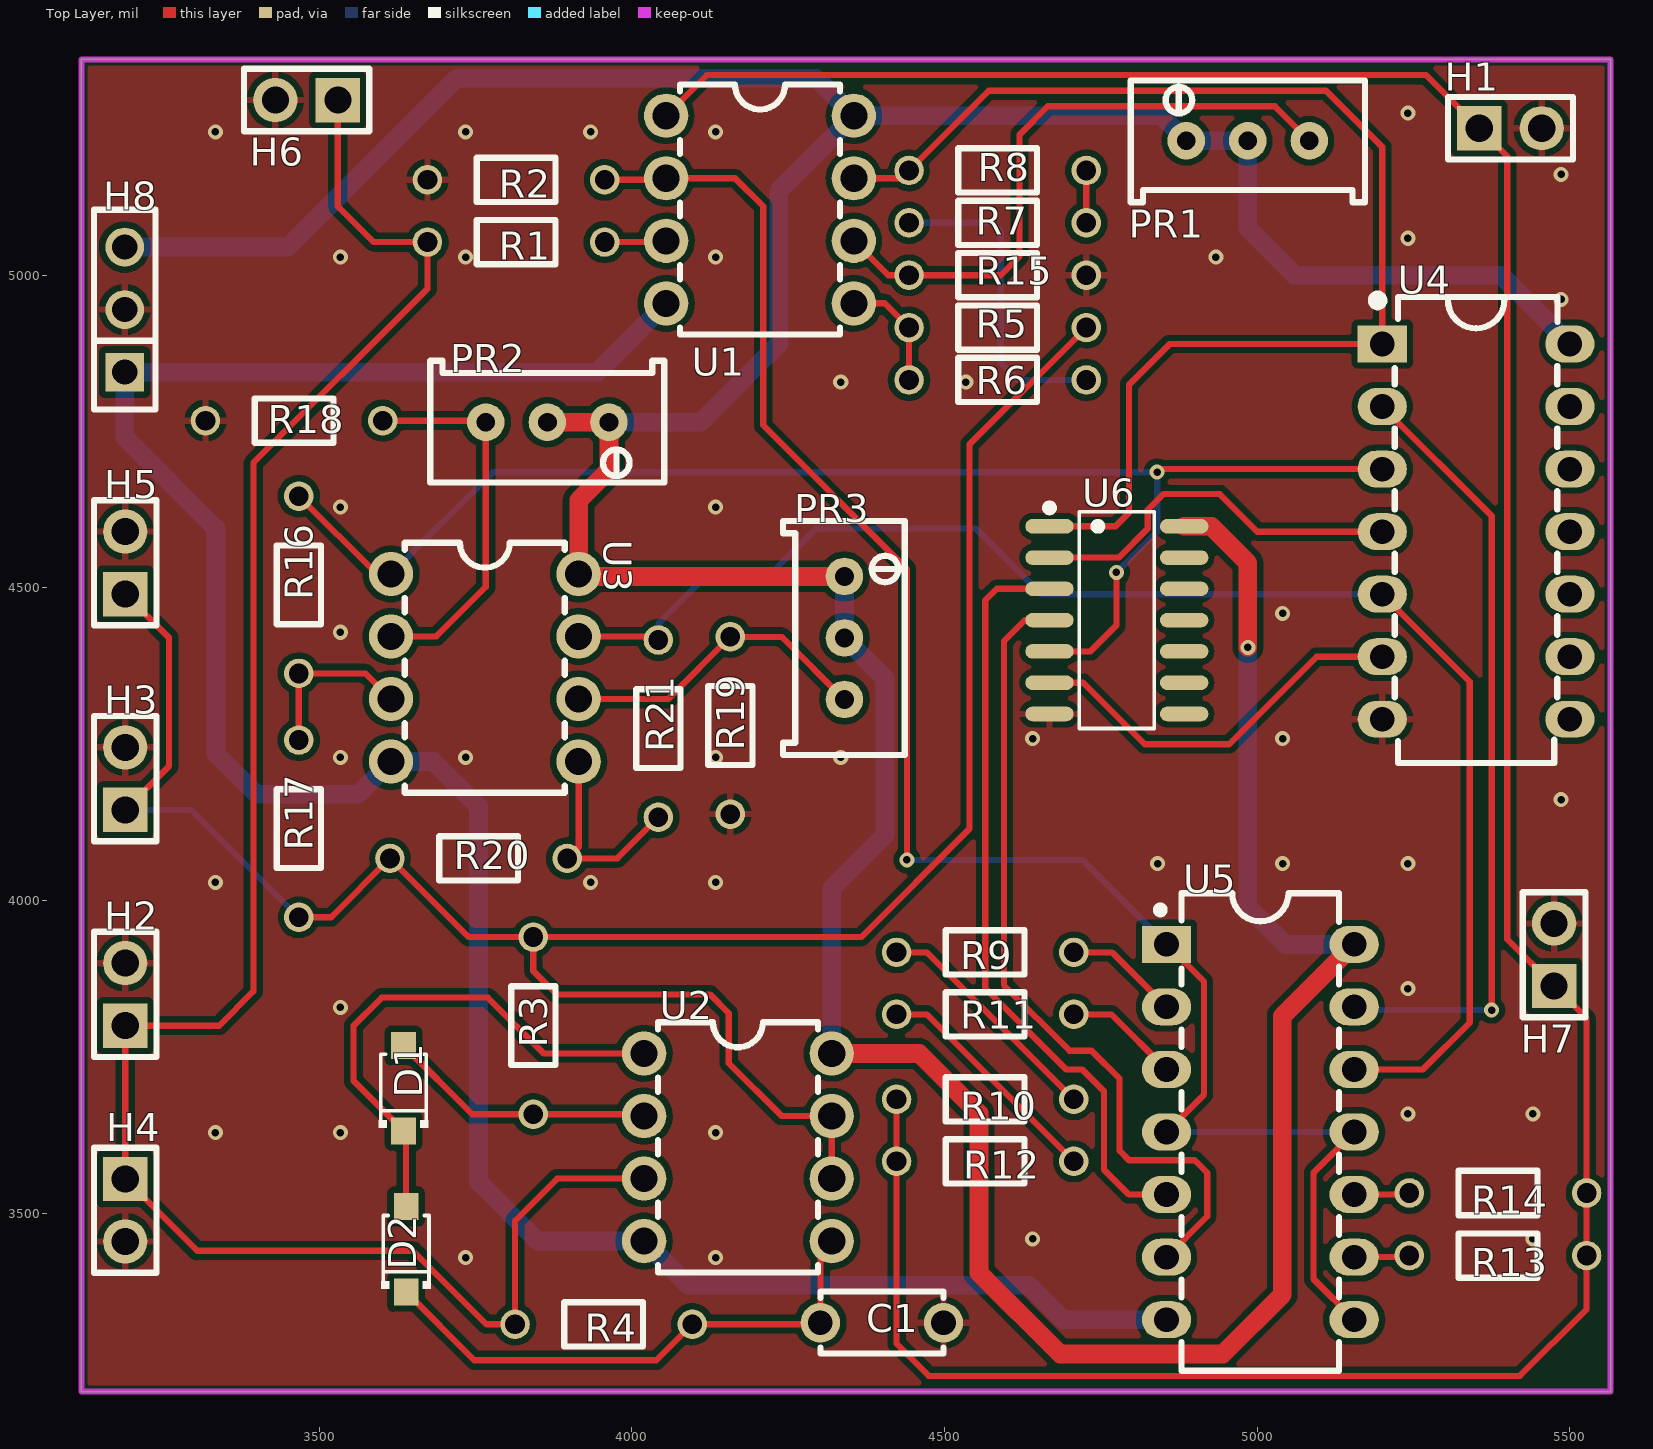
[diagram p0: Top Layer view]
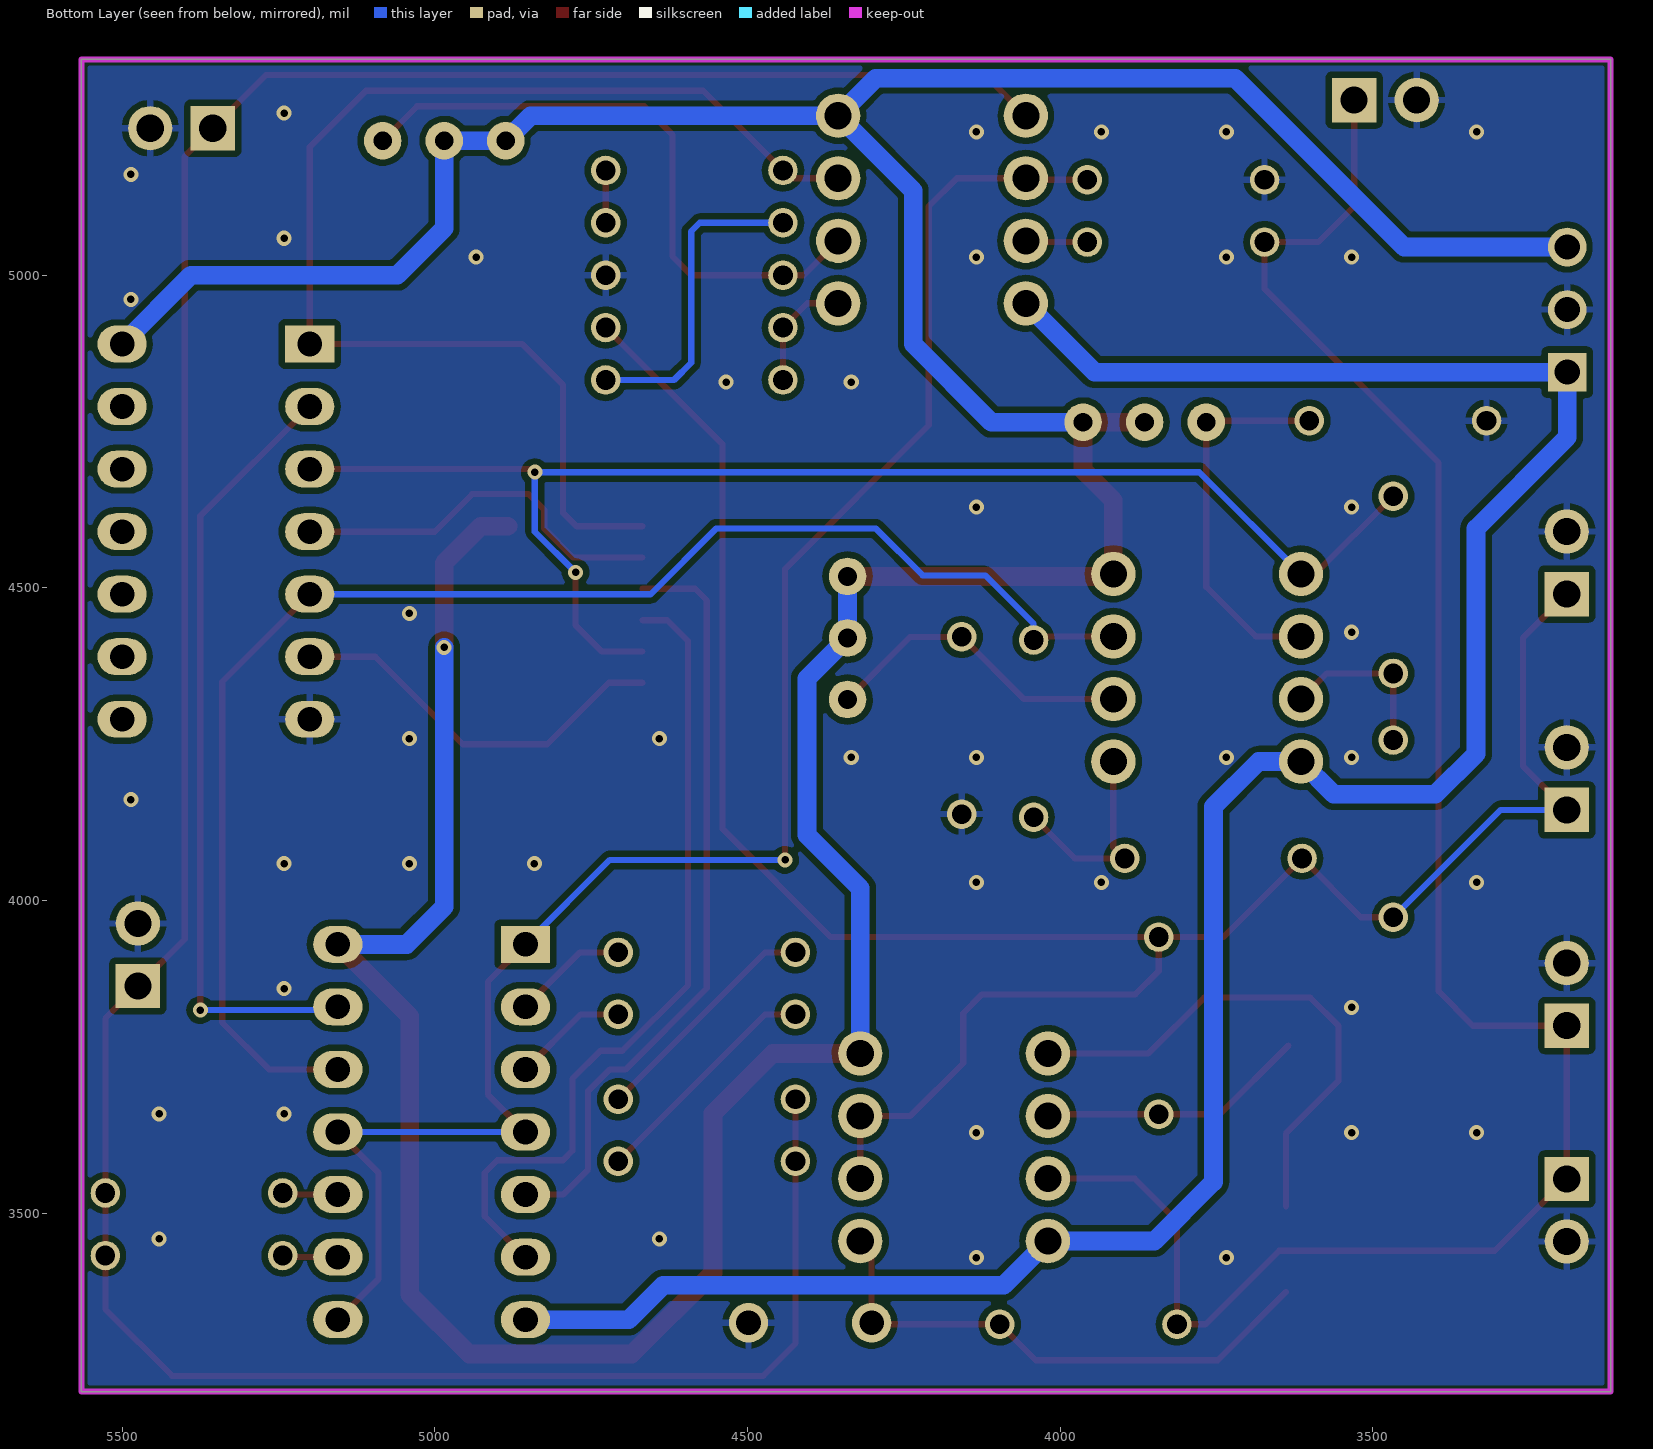
[diagram p1: Bottom Layer view, seen from below]
# Altium PCB MISC51795.pcbdoc
Units mil, origin at the board's own origin, x right, y up, seen from the top; angles counter-clockwise.
Board outline 2445 x 2130 mil, 2 copper layers (Top Layer, Bottom Layer), stack 62.206 mil thick; 41 components, 39 nets, 140 pads, 47 vias.

## Layer stack, top to bottom
Top Solder Mask Layer: solder mask 0.394, Dk 3.3
Top Layer: signal copper 1.379
Dielectric1: surface 59.449, FR4, Dk 4.5
Bottom Layer: signal copper 1.378
Bottom Solder Mask Layer: solder mask 0.394, Dk 3.3

## Board outline
3120,5345 3120,3215 5565,3215 5565,5345

## Design rules (kind name [scope] priority, off if disabled: settings)
BoardOutlineClearance copperThickness2oz_1 [All] p2 off: genericclearance=7.99 ignorepadtopadclearanceinfootprint=FALSE except(0: Arc-SplitContinuation Track-SplitContinuation SMDPad-SplitContinuation THPad-SplitContinuation Via-SplitContinuation Fill-SplitContinuation Region-SplitContinuation Poly-SplitContinuation Text-SplitContinuation Hole-SplitContinuation; 5.98: Arc-CutoutEdge SMDPad-CutoutEdge THPad-CutoutEdge Via-CutoutEdge Fill-CutoutEdge Region-CutoutEdge Text-CutoutEdge; 6.93: Hole-OutlineEdge Hole-CutoutEdge; 10: Poly-OutlineEdge Poly-CutoutEdge; 11.81: Arc-OutlineEdge Track-OutlineEdge SMDPad-OutlineEdge THPad-OutlineEdge Via-OutlineEdge Fill-OutlineEdge Region-OutlineEdge Text-OutlineEdge Track-CutoutEdge)
BoardOutlineClearance copperThickness1oz_1 [All] p4: genericclearance=4.02 ignorepadtopadclearanceinfootprint=FALSE except(0: Arc-SplitContinuation Track-SplitContinuation SMDPad-SplitContinuation THPad-SplitContinuation Via-SplitContinuation Fill-SplitContinuation Region-SplitContinuation Poly-SplitContinuation Text-SplitContinuation Hole-SplitContinuation; 6: SMDPad-CutoutEdge THPad-CutoutEdge Via-CutoutEdge Fill-CutoutEdge Region-CutoutEdge Text-CutoutEdge; 6.93: Hole-OutlineEdge Hole-CutoutEdge; 10: Poly-OutlineEdge Poly-CutoutEdge; 11.8: Arc-OutlineEdge Track-OutlineEdge SMDPad-OutlineEdge THPad-OutlineEdge Via-OutlineEdge Fill-OutlineEdge Region-OutlineEdge Text-OutlineEdge; 11.81: Arc-CutoutEdge Track-CutoutEdge)
Clearance copperThickness2oz [All] p1 off: gap=7.99 ignorepadtopadclearanceinfootprint=FALSE except(5.98: SMDPad-Track SMDPad-SMDPad THPad-Track SMDPad-THPad THPad-THPad Track-Via SMDPad-Via THPad-Via Via-Via Fill-Track Region-Track Fill-SMDPad Region-SMDPad Fill-THPad Region-THPad Fill-Via Region-Via Fill-Fill Fill-Region Region-Region Arc-Track Arc-SMDPad Arc-THPad Arc-Via Fill-Arc Region-Arc Arc-Arc Text-Track SMDPad-Text Text-THPad Text-Via Fill-Text Region-Text Arc-Text Text-Text; 6.93: Hole-Track Hole-SMDPad Hole-THPad Hole-Via Fill-Hole Region-Hole Hole-Arc Hole-Text; 10: Poly-Track Poly-SMDPad Poly-THPad Poly-Via Poly-Fill Poly-Region Poly-Poly Poly-Arc Poly-Text Poly-Hole)
Clearance copperThickness1oz [All] p3: gap=4.02 ignorepadtopadclearanceinfootprint=FALSE except(5.98: SMDPad-Track SMDPad-SMDPad THPad-Track SMDPad-THPad THPad-THPad Track-Via SMDPad-Via THPad-Via Via-Via Fill-Track Region-Track Fill-SMDPad Region-SMDPad Fill-THPad Region-THPad Fill-Via Region-Via Fill-Fill Fill-Region Region-Region; 6: Arc-Track Arc-SMDPad Arc-THPad Arc-Via Fill-Arc Region-Arc Arc-Arc Text-Track SMDPad-Text Text-THPad Text-Via Fill-Text Region-Text Arc-Text Text-Text; 6.93: Hole-Track Hole-SMDPad Hole-THPad Hole-Via Fill-Hole Region-Hole Hole-Arc Hole-Text; 10: Poly-Track Poly-SMDPad Poly-THPad Poly-Via Poly-Fill Poly-Region Poly-Poly Poly-Arc Poly-Text Poly-Hole)
Creepage creepage [All] p1: checkdistance=0 ignoreinternallayers=TRUE applytopolygonpour=TRUE
DiffPairsRouting differentialPair [All] p1: maxlimit=6 minlimit=6 mostfreqgap=6 toplayer_minwidth=5 toplayer_prefwidth=10 toplayer_maxwidth=100 toplayer_mingap=6 toplayer_prefgap=6 toplayer_maxgap=6 bottomlayer_minwidth=5 bottomlayer_prefwidth=10 bottomlayer_maxwidth=100 bottomlayer_mingap=6 bottomlayer_prefgap=6 bottomlayer_maxgap=6 maxuncoupledlength=10
HoleToHoleClearance otherClearance [All] p1: gap=11.81 allowstackedmicrovias=TRUE
Length netLength [All] p1: minlimit=0 maxlimit=0
MatchedLengths netLengthTolerance [All] p1: tolerance=1000
PasteMaskExpansion pasteMaskExpansion [All] p1: expansion=0
PlaneConnect innerPlane [All] p1: planeconnectstyle=Relief reliefexpansion=20 reliefentries=4 reliefconductorwidth=10 reliefairgap=10
PolygonConnect copperRegion [(InNet('GND'))] p1: connectstyle=Relief reliefconductorwidth=10 reliefentries=4 polygonreliefangle="90 Angle" airgapwidth=10 via.connectstyle=Relief via.reliefconductorwidth=10 via.reliefentries=4 via.polygonreliefangle="90 Angle" via.airgapwidth=10
RoutingVias viaSize [All] p1: holewidth=12.01 width=24.02 viastyle="Through Hole" minholewidth=11.81 minwidth=19.68 maxholewidth=248.03 maxwidth=393.7
SolderMaskExpansion solderMaskExpansion [IsVia] p1: expansion=-1000 istentingtop=TRUE
SolderMaskExpansion solderMaskExpansion [All] p2: expansion=2 istentingtop=FALSE
Width copperThickness2oz_2 [All] p1 off: maxlimit=100 minlimit=8 preferedwidth=10
Width copperThickness1oz_2 [All] p2: maxlimit=100 minlimit=5 preferedwidth=10

## Components (designator, comment, footprint, x,y, rotation, side; value= is the part's Value field where it differs from the comment)
C1 "22uF" CAP-TH_L5.0-W2.5-P5.00-D1.0 4400,3325 r180 top
D1 "1N4148W" SOD-123F_L2.7-W1.6-LS3.8-RD 3635,3700 r90 top
D2 "1N4148W" SOD-123F_L2.7-W1.6-LS3.8-RD 3639.08,3442.49 r90 top
H1 "" HDR-TH_2P-P2.54-V-M-1 5405,5235 r0 top
H2 "" HDR-TH_2P-P2.54-V-M-1 3190,3850.04 r90 top
H3 "" HDR-TH_2P-P2.54-V-M-1 3190,4195.08 r90 top
H4 "" HDR-TH_2P-P2.54-V-M-1 3190,3505 r270 top
H5 "" HDR-TH_2P-P2.54-V-M-1 3190,4540.12 r90 top
H6 "" HDR-TH_2P-P2.54-V-M-1 3480,5280 r180 top
H7 "" HDR-TH_2P-P2.54-V-M-1 5474.79,3913.46 r90 top
H8 "" HDR-TH_3P-P2.54-V-F 3189.21,4945 r90 top
PR1 "51kΩ" R_3296 4985,5220 r0 top
PR2 "51kΩ" R_3296 3865,4760 r180 top
PR3 "51kΩ" R_3296 4345,4420 r270 top
R1 "10K" Res_1/8W 3815,5050.47 r0 top
R2 "10K" Res_1/8W 3815,5150 r0 top
R3 "1K" Res_1/8W 3845,3800 r90 top
R4 "10K" Res_1/8W 3955,3320 r0 top
R5 "1K" Res_1/8W 4585,4918.71 r180 top
R6 "100K" Res_1/8W 4585,4830 r0 top
R7 "82K" Res_1/8W 4585,5081.29 r0 top
R8 "5.1K" Res_1/8W 4585,5170 r180 top
R9 "45K" Res_1/8W 4565.05,3919.68 r180 top
R10 "5.1K" Res_1/8W 4565.05,3684.68 r180 top
R11 "39K" Res_1/8W 4565.05,3820.56 r180 top
R12 "1K" Res_1/8W 4565.05,3585.56 r180 top
R13 "20K" Res_1/8W 5385,3430 r0 top
R14 "9.5K" Res_1/8W 5385,3530 r0 top
R15 "2K" Res_1/8W 4585,5002.48 r180 top
R16 "75K" Res_1/8W 3470,4505 r90 top
R17 "1K" Res_1/8W 3470,4115 r90 top
R18 "2K" Res_1/8W 3460,4765 r0 top
R19 "2K" Res_1/8W 4160,4280 r90 top
R20 "1K" Res_1/8W 3755,4065 r0 top
R21 "75K" Res_1/8W 4045,4275 r90 top
U1 "LM358AP" PDIP-8_L10.2-W6.5-P2.54-LS7.6-BL 4205,5105 r270 top
U2 "LM358AN/NOPB" PDIP-8_L10.2-W6.5-P2.54-LS7.6-BL 4169.69,3605.56 r270 top
U3 "LM358AN/NOPB" PDIP-8_L10.2-W6.5-P2.54-LS7.6-BL 3765,4372.38 r270 top
U4 "CD40106BD" DIP-14_L19.1-W6.4-P2.54-LS7.6-BL 5350,4590 r270 top
U5 "SN74LV4066AN" PDIP-14_L19.3-W6.4-P2.54-LS7.9-BL-1 5005,3630 r270 top
U6 "HEF4081BT118" SO-14_L8.9-W3.9-P1.27-LS6.0-BL 4775.51,4448.46 r270 top

## Footprints (in the part's own frame and the unit in brackets; to place one, negate y for a bottom-side part, rotate by r counter-clockwise, add the part's x,y. Pads: shape width x height; smd on the part's side, far side on the other; paste and mask are expansions set on the pad)
CAP-TH_L5.0-W2.5-P5.00-D1.0 [mm]
  round 1.6 hole 1: 1(-2.5,0) 2(2.5,0)
  silkscreen extent -2.5,-1.27 2.5,1.25
DIP-14_L19.1-W6.4-P2.54-LS7.6-BL [mm]
  rect 1.5x2 hole 1: 1(-7.62,-3.81)
  oval 1.5x2 hole 1: 2(-5.08,-3.81) 3(-2.54,-3.81) 4(0,-3.81) 5(2.54,-3.81) 6(5.08,-3.81) 7(7.62,-3.81) 8(7.62,3.81) 9(5.08,3.81) 10(2.54,3.81) 11(0,3.81) 12(-2.54,3.81) 13(-5.08,3.81) 14(-7.62,3.81)
  silkscreen extent -9.59,-4.2 9.4,3.3
HDR-TH_2P-P2.54-V-M-1 [mm]
  rect 1.8x1.8 hole 1.1: 1(-1.27,0)
  round 1.8 hole 1.1: 2(1.27,0)
  silkscreen extent -2.54,-1.27 2.54,1.27
HDR-TH_3P-P2.54-V-F [mil]
  rect 62x62 hole 40.16: 1(-100,0)
  round 62 hole 40.16: 2(0,0) 3(100,0)
  silkscreen extent -160,-49 160,49
PDIP-8_L10.2-W6.5-P2.54-LS7.6-BL [mm]
  round 1.8 hole 1.1: 1(-3.81,-3.81) 2(-1.27,-3.81) 3(1.27,-3.81) 4(3.81,-3.81) 5(3.81,3.81) 6(1.27,3.81) 7(-1.27,3.81) 8(-3.81,3.81)
  silkscreen extent -5.08,-3.25 5.08,3.25
PDIP-14_L19.3-W6.4-P2.54-LS7.9-BL-1 [mm]
  rect 1.5x2 hole 1: 1(-7.62,-3.81)
  oval 1.5x2 hole 1: 2(-5.08,-3.81) 3(-2.54,-3.81) 4(0,-3.81) 5(2.54,-3.81) 6(5.08,-3.81) 7(7.62,-3.81)
  oval 1.5x2 hole 1 copper offset 0,0: 8(7.62,3.81) 9(5.08,3.81) 10(2.54,3.81) 11(0,3.81) 12(-2.54,3.81) 13(-5.08,3.81) 14(-7.62,3.81)
  silkscreen extent -9.7,-4.21 9.7,3.2
R_3296 [mil]
  round 60 hole 30 paste+0 mask+2: 1(-98.4,-5) 2(0,-5) 3(98.4,-5)
  silkscreen extent -187,-103 187,92
Res_1/8W [mil]
  round 47.2 hole 31.5 paste+0 mask+2: 1(-141.7,2.48) 2(141.7,2.48)
  silkscreen extent -63,-33 63,38
SO-14_L8.9-W3.9-P1.27-LS6.0-BL [mm]
  oval 0.595x1.968 smd: 1(-3.81,-2.734) 2(-2.54,-2.734) 3(-1.27,-2.734) 4(0,-2.734) 5(1.27,-2.734) 6(2.54,-2.734) 7(3.81,-2.734) 8(3.81,2.734) 9(2.54,2.734) 10(1.27,2.734) 11(0,2.734) 12(-1.27,2.734) 13(-2.54,2.734) 14(-3.81,2.734)
  silkscreen extent -4.71,-2.88 4.4,1.52
SOD-123F_L2.7-W1.6-LS3.8-RD [mm]
  rect 1.1x1 smd: 1(-1.735,0) 2(1.735,0)
  silkscreen extent -1.6,-1 1.38,1

## Via types
v1: diameter 24.02, hole 12, Top Layer to Bottom Layer, 47 vias

## Nets (pads, with @x,y where several pads share a name; then routed paths per layer and width w, separated by ;. In a path a pad name is that pad's centre, name@x,y a point inside that pad or via, vN(x,y) a via of type N, cw(c..) or ccw(c..) an arc to the next point about the centre after c; other vN are vias at no path point)
9V: H8.3 PR1.1 PR1.2 PR2.1 PR2.2 PR3.1 PR3.2 U1.8 U2.8 U3.8 U4.14 U5.14 U6.14 | length 7618.2
  Top Layer w30: PR2.2 PR2.1 3963.4,4688.4 3915,4640 U3.8 3918.98,4518.4 PR3.1 ; U2.8 4459.44,3755.56 4555,3660 4555,3405 4685,3275 4945,3275 5040,3370 5040,3815 U5.14 ; U6.14 4926.54,4598.46 4985,4540 v1(4985,4405)
  Bottom Layer w30: H8.3 3450,5045 3720,5315 4295,5315 U1.8 ; PR2.1 4110,4765 4235,4890 4235,5135 U1.8 ; U2.8 4319.69,4019.68 4405,4105 4405,4355 PR3.2 PR3.1 ; v1(4985,4405) 4985,3990 5045,3930 U5.14 ; U4.14 5390,5000 5060,5000 4985,5075 PR1.2 PR1.1 4846.6,5255 U1.8
$1N4: R1.2 U1.3 | length 99.2
  Top Layer w10: R1.2 4052.95,5052.95 U1.3
$1N7: H2.1 H4.1 H6.1 R1.1 R4.1 U2.3 | length 3242.6
  Top Layer w10: H6.1 3530,5110 3587.05,5052.95 R1.1 3673.3,4978.3 3395,4700 3395,3855 3340.04,3800.04 H2.1 H4.1 3305,3440 3650,3440 3767.52,3322.48 R4.1 3813.3,3488.3 3880.56,3555.56 U2.3
$1N12: D1.2 R3.1 U2.2 | length 431.4
  Top Layer w10: D1.2 3745.01,3658.3 R3.1 4016.94,3658.3 U2.2
$1N13: D1.1 D2.2 U2.1 | length 844.4
  Top Layer w10: D2.2 3639.08,3627.62 D1.1 3555,3711.7 3555,3800 3600,3845 3770,3845 3859.44,3755.56 U2.1
$1N14: C1.2 D2.1 R4.2 U2.5 | length 870.6
  Top Layer w10: D2.1 3748.26,3265 4039.22,3265 R4.2 4299.05,3322.48 C1.2 4301.57,3437.45 U2.5
$1N21: R5.2 R6.1 U1.5 | length 188.1
  Top Layer w10: U1.5 4404.54,4955 R5.2 R6.1
$1N22: R6.2 R7.1 | length 510.5
  Bottom Layer w10: R7.1 4576.24,5083.76 4590,5070 4590,4860 4617.52,4832.48 R6.2
$1N24: R7.2 R8.1 | length 83.8
  Top Layer w10: R7.2 R8.1
$1N26: PR1.3 R15.2 U1.6 | length 1000
  Top Layer w10: U1.6 4410,5000 R15.2 4590,5000 4620,5030 4620,5225 4665,5270 5028.4,5270 PR1.3
$1N44: R2.2 U1.2 U5.1 U5.4 U5.8 U5.11 | length 2887.7
  Top Layer w10: R2.2 4052.48,5152.48 U1.2 4165,5155 4210,5110 4210,4760 4440,4530 v1(4440,4065) ; U5.4 4915,3690 4915,3870.01 U5.1 ; U5.8 5090,3395 5090,3565 U5.11
  Bottom Layer w10: v1(4440,4065) 4720.01,4065 U5.1 ; U5.4 U5.11
$1N45: U5.5 U6.3 | length 1230.4
  Top Layer w10: U6.3 4583.46,4498.46 4565,4480 4565,3860 4695,3730 4720,3730 4755,3695 4755,3570 4795,3530 U5.5
$1N47: R9.1 U5.2 | length 184.4
  Top Layer w10: R9.1 4767.79,3917.21 U5.2
$1N48: R9.2 R10.1 | length 380.7
  Top Layer w10: R9.2 4471.75,3917.21 R10.1
$1N49: R11.2 R12.1 | length 380.7
  Top Layer w10: R11.2 4471.75,3818.08 R12.1
$1N50: R11.1 U5.3 | length 184.7
  Top Layer w10: R11.1 4766.92,3818.08 U5.3
$1N51: R13.1 U5.9 | length 89.3
  Top Layer w10: U5.9 5240.82,3430 R13.1
$1N52: R14.1 U5.10 | length 89.3
  Top Layer w10: U5.10 5240.82,3530 R14.1
$1N56: H1.1 H7.1 R10.2 R12.2 R13.2 R14.2 U1.1 | length 4881.1
  Top Layer w10: U1.1 4120,5320 5270,5320 H1.1 5400,5190 5400,3938.26 H7.1 5526.7,3811.56 R14.2 R13.2 5526.7,3346.7 5420,3240 4475,3240 4423.35,3291.65 R12.2 R10.2
$1N62: R16.1 R17.2 U3.3 | length 271
  Top Layer w10: R17.2 R16.1 3574.08,4363.3 U3.3
$1N67: PR2.3 R18.2 U3.2 | length 613.7
  Top Layer w10: R18.2 3764.12,4767.48 PR2.3 3766.6,4501.6 3687.38,4422.38 U3.2
$1N73: R20.2 R21.1 U3.5 | length 335.6
  Top Layer w10: U3.5 3915,4085.77 R20.2 3976.7,4067.48 R21.1
$1N74: H3.1 H5.1 R3.2 R5.1 R17.1 R20.1 U2.6 U2.7 | length 3640
  Top Layer w10: H3.1 3260,4215.08 3260,4420.12 H5.1 ; R17.1 3519.12,3973.3 R20.1 3739.08,3941.7 R3.2 ; U2.6 U2.7 4239.44,3655.56 4155,3740 4155,3820 4125,3850 3880,3850 3842.52,3887.48 R3.2 ; R5.1 4540,4729.54 4540,4115 4366.7,3941.7 R3.2
  Bottom Layer w10: H3.1 3295.74,4145.08 R17.1
$1N75: PR3.3 R19.2 U3.6 | length 507.6
  Top Layer w10: U3.6 4058.21,4322.38 R19.2 4239.9,4421.7 PR3.3
$1N76: U5.6 U6.4 | length 1315.3
  Top Layer w10: U6.4 4628.46,4448.46 4595,4415 4595,3865 4700,3760 4735,3760 4780,3715 4780,3600 4795,3585 4900,3585 4920,3565 4920,3495 U5.6
-9V: H8.1 U1.4 U2.4 U3.4 U5.7 | length 3871.5
  Bottom Layer w30: U1.4 3945,4845 H8.1 3189.21,4740.79 3335,4595 3335,4235 3400,4170 3562.61,4170 U3.4 3682.62,4222.38 3755,4150 3755,3550 3849.44,3455.56 U2.4 4090.24,3385 4635,3385 4690,3330 U5.7
GND: C1.1 H1.2 H2.2 H3.2 H4.2 H5.2 H6.2 H7.2 H8.2 R2.1 R15.1 R18.1 R19.1 U4.7 U6.7
  other v1: 3734.1,3429.1 4134.1,3429.1 4640.79,3459.1 5440.79,3459.1 3334.1,3629.1 3534.1,3629.1 4134.1,3629.1 5240.79,3659.1 5440.79,3659.1 3534.1,3829.1 5240.79,3859.1 3334.1,4029.1 3934.1,4029.1 4134.1,4029.1 4840.79,4059.1 5040.79,4059.1 5240.79,4059.1 5486.11,4161.38 3534.1,4229.1 3734.1,4229.1 4134.1,4229.1 4334.1,4229.1 4640.79,4259.1 5040.79,4259.1 3534.1,4429.1 5040.79,4459.1 3534.1,4629.1 4134.1,4629.1 4334.1,4829.1 4534.1,4829.1 5486.11,4961.38 3534.1,5029.1 3734.1,5029.1 4134.1,5029.1 4934.1,5029.1 5240.79,5059.1 5486.11,5161.38 3334.1,5229.1 3734.1,5229.1 3934.1,5229.1 4134.1,5229.1 5240.79,5259.1
IN1: R8.2 U1.7 U4.1 U6.1 | length 2028.2
  Top Layer w10: U1.7 4430.78,5155 R8.2 4570.78,5295 5110,5295 5200,5205 U4.1 4860,4890 4795,4825 4795,4620 4773.46,4598.46 U6.1
IN2: R16.2 U3.1 U4.3 U6.5 | length 2249.6
  Top Layer w10: R16.2 3591.84,4522.38 U3.1 ; U6.5 4733.46,4398.46 4775,4440 v1(4775,4525) ; v1(4840,4685) 4845,4690 U4.3
  Bottom Layer w10: U3.1 3777.61,4685 v1(4840,4685) 4840,4590 v1(4775,4525)
IN3: R21.2 U3.7 U4.5 U5.12 | length 2378.9
  Top Layer w10: U3.7 4036.84,4422.38 R21.2 ; U5.12 5265,3730 5340,3805 5340,4350 U4.5
  Bottom Layer w10: R21.2 4042.52,4442.52 4120,4520 4220,4520 4295,4595 4550,4595 4655,4490 U4.5
IN4: U4.9
IN5: U4.11
IN6: U4.13
OUT1: U4.2 U5.13 | length 1259.6
  Top Layer w10: U4.2 5375,4615 v1(5375,3825)
  Bottom Layer w10: U5.13 5160,3825 v1(5375,3825)
OUT2: U4.4 U6.2 | length 616.6
  Top Layer w10: U6.2 4778.46,4548.46 4825,4595 4825,4625 4850,4650 4940,4650 5000,4590 U4.4
OUT3: U4.6 U6.6 | length 630.9
  Top Layer w10: U6.6 4721.54,4348.46 4820,4250 4955,4250 5095,4390 U4.6
OUT4: U4.8
OUT5: U4.10
OUT6: U4.12
pads on no net: U6.8 U6.9 U6.10 U6.11 U6.12 U6.13

## Polygon pours and split planes (outlines as drawn)
GND on Bottom Layer (solid, remove dead copper, pour order 2): 3000,5520 3000,3000 5740,3000 5740,5520
GND on Top Layer (solid, remove dead copper, pour order 0): 3030,5460 3030,3100 5850,3100 5850,5460

## Keep-outs
Board Outline Layer:
  the board outline again, w10